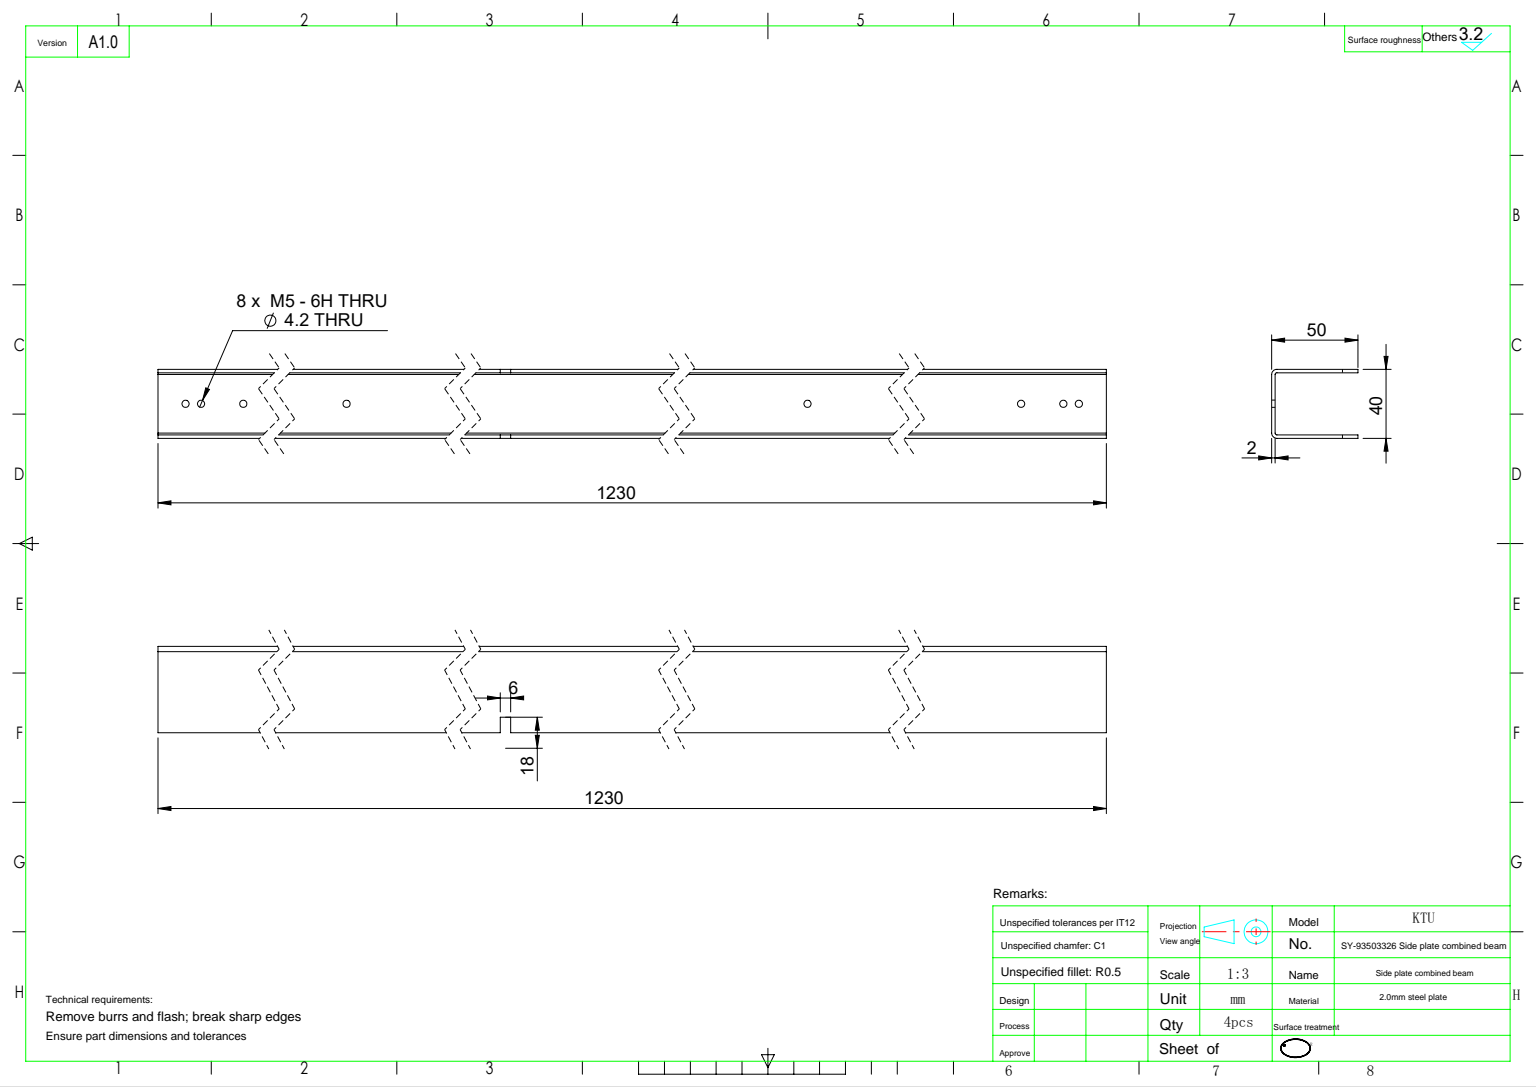
from build123d import *

# Parameters (mm, degrees)
EXTRUDE_1_DEPTH     = 615
SKETCH_2_W          = 18
SKETCH_2_H          = 6
CUT_EXTRUDE_1_DEPTH = 617.8062905
HOLE_WIZARD_M5_1_D  = 4.2


with BuildPart() as part:
    # 草图1 → 拉伸-薄壁1 (new, symmetric)
    with BuildSketch(Plane.XY):
        with BuildLine():
            Line((25, -20), (-22, -20))
            ThreePointArc((-22, -20), (-24.121320344, -19.121320344), (-25, -17))
            Line((-25, -17), (-25, 17))
            ThreePointArc((-25, 17), (-24.121320344, 19.121320344), (-22, 20))
            Line((-22, 20), (25, 20))
            Line((25, 20), (25, 18))
            Line((25, 18), (-22, 18))
            ThreePointArc((-22, 18), (-22.707106781, 17.707106781), (-23, 17))
            Line((-23, 17), (-23, -17))
            ThreePointArc((-23, -17), (-22.707106781, -17.707106781), (-22, -18))
            Line((-22, -18), (25, -18))
            Line((25, -18), (25, -20))
        make_face()
    extrude(amount=EXTRUDE_1_DEPTH, both=True)

    # 草图2 → 切除-拉伸1 (cut, through all)
    with BuildSketch(Plane.XZ.offset(20)):
        with Locations((25, 45)):
            Rectangle(SKETCH_2_W, SKETCH_2_H)
    extrude(amount=-CUT_EXTRUDE_1_DEPTH, mode=Mode.SUBTRACT)

    # M5 螺纹孔1 (through all)
    with Locations(Plane.ZY.offset(25)):
        with Locations((590, 0), (320, 0), (-320, 0), (-590, 0), (565.5, 0), (599, 0), (-599, 0), (-565.5, 0)):
            Hole(HOLE_WIZARD_M5_1_D / 2)


solid = part.part
